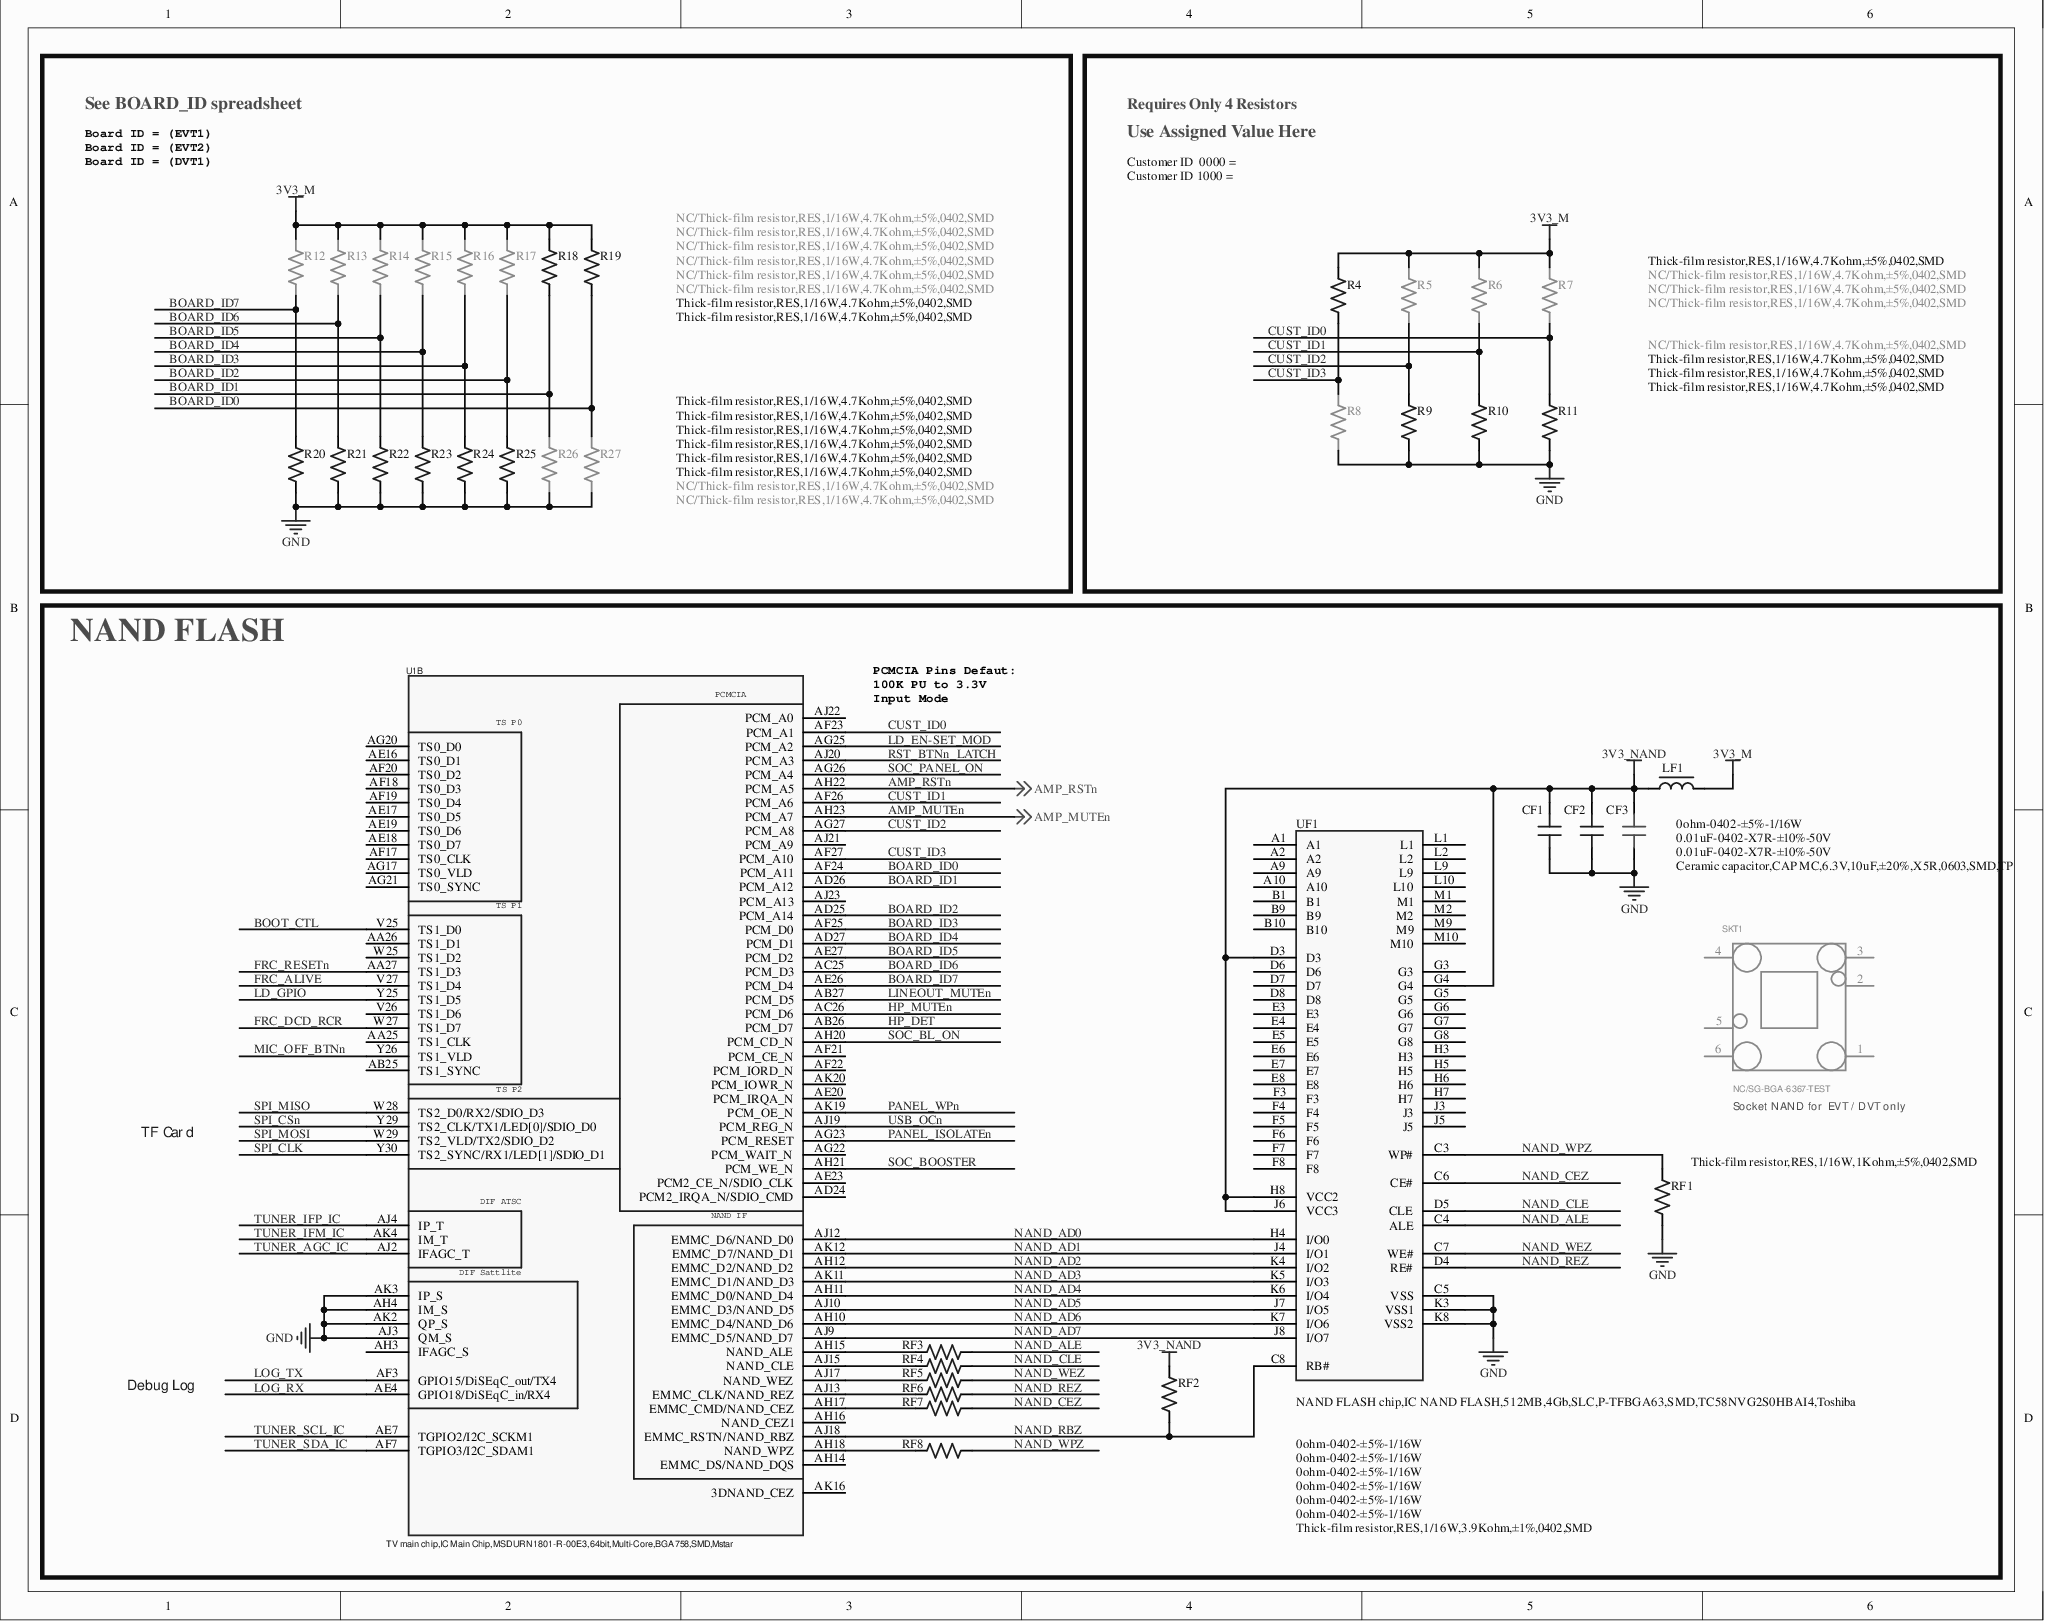
[diagram p0: MISC86290-10.SchDoc]
# Altium project MISC86290.PrjPcb (part 8 of 13)

## Sheet MISC86290-10.SchDoc
size 368 x 292 mm

### Parts
CF1  0.01uF-0402-X7R-±10%-50V  [C0402]
CF2  0.01uF-0402-X7R-±10%-50V  [C0402]
CF3  Ceramic capacitor,CAP MC,6.3V,10uF,±20%,X5R,0603,SMD,TP  [C0603]
LF1  0ohm-0402-±5%-1/16W  [L0402]
R4  Thick-film resistor,RES,1/16W,4.7Kohm,±5%,0402,SMD  [R0402]
R5  NC/Thick-film resistor,RES,1/16W,4.7Kohm,±5%,0402,SMD  [R0402]
R6  NC/Thick-film resistor,RES,1/16W,4.7Kohm,±5%,0402,SMD  [R0402]
R7  NC/Thick-film resistor,RES,1/16W,4.7Kohm,±5%,0402,SMD  [R0402]
R8  NC/Thick-film resistor,RES,1/16W,4.7Kohm,±5%,0402,SMD  [R0402]
R9  Thick-film resistor,RES,1/16W,4.7Kohm,±5%,0402,SMD  [R0402]
R10  Thick-film resistor,RES,1/16W,4.7Kohm,±5%,0402,SMD  [R0402]
R11  Thick-film resistor,RES,1/16W,4.7Kohm,±5%,0402,SMD  [R0402]
R12  NC/Thick-film resistor,RES,1/16W,4.7Kohm,±5%,0402,SMD  [R0402]
R13  NC/Thick-film resistor,RES,1/16W,4.7Kohm,±5%,0402,SMD  [R0402]
R14  NC/Thick-film resistor,RES,1/16W,4.7Kohm,±5%,0402,SMD  [R0402]
R15  NC/Thick-film resistor,RES,1/16W,4.7Kohm,±5%,0402,SMD  [R0402]
R16  NC/Thick-film resistor,RES,1/16W,4.7Kohm,±5%,0402,SMD  [R0402]
R17  NC/Thick-film resistor,RES,1/16W,4.7Kohm,±5%,0402,SMD  [R0402]
R18  Thick-film resistor,RES,1/16W,4.7Kohm,±5%,0402,SMD  [R0402]
R19  Thick-film resistor,RES,1/16W,4.7Kohm,±5%,0402,SMD  [R0402]
R20  Thick-film resistor,RES,1/16W,4.7Kohm,±5%,0402,SMD  [R0402]
R21  Thick-film resistor,RES,1/16W,4.7Kohm,±5%,0402,SMD  [R0402]
R22  Thick-film resistor,RES,1/16W,4.7Kohm,±5%,0402,SMD  [R0402]
R23  Thick-film resistor,RES,1/16W,4.7Kohm,±5%,0402,SMD  [R0402]
R24  Thick-film resistor,RES,1/16W,4.7Kohm,±5%,0402,SMD  [R0402]
R25  Thick-film resistor,RES,1/16W,4.7Kohm,±5%,0402,SMD  [R0402]
R26  NC/Thick-film resistor,RES,1/16W,4.7Kohm,±5%,0402,SMD  [R0402]
R27  NC/Thick-film resistor,RES,1/16W,4.7Kohm,±5%,0402,SMD  [R0402]
RF1  Thick-film resistor,RES,1/16W,1Kohm,±5%,0402,SMD  [R0402]
RF2  Thick-film resistor,RES,1/16W,3.9Kohm,±1%,0402,SMD  [R0402]
RF3  0ohm-0402-±5%-1/16W  [R0402]
RF4  0ohm-0402-±5%-1/16W  [R0402]
RF5  0ohm-0402-±5%-1/16W  [R0402]
RF6  0ohm-0402-±5%-1/16W  [R0402]
RF7  0ohm-0402-±5%-1/16W  [R0402]
RF8  0ohm-0402-±5%-1/16W  [R0402]
SKT1  NC/SG-BGA-6367-TEST  [TEST-SG-BGA-6367]
U1  TV main chip,IC Main Chip,MSDURN1801-R-00E3,64bit,Multi-Core,BGA758,SMD,Mstar  [BGA758/0.65]  (part B of 7)
UF1  NAND FLASH chip,IC NAND FLASH,512MB,4Gb,SLC,P-TFBGA63,SMD,TC58NVG2S0HBAI4,Toshiba  [BGA63/0.8-1]

### Blocks framed on the sheet
See BOARD_ID spreadsheet: R12-R27
Use Assigned Value Here: R4-R11
NAND FLASH: CF1-CF3 LF1 RF1-RF8 SKT1 U1 UF1

### Nets
3V3_M: LF1.2 R4.2 R5.2 R6.2 R7.2 R12.2 R13.2 R14.2 R15.2 R16.2 R17.2 R18.2 R19.2
3V3_NAND: CF1.2 CF2.2 CF3.2 LF1.1 RF2.2 UF1.D3 UF1.G4 UF1.H8(VCC2) UF1.J6(VCC3)
GND: CF1.1 CF2.1 CF3.1 R8.1 R9.1 R10.1 R11.1 R20.1 R21.1 R22.1 R23.1 R24.1 R25.1 R26.1 R27.1 RF1.1 U1.AH4(IM_S) U1.AJ3(QM_S) U1.AK2(QP_S) U1.AK3(IP_S) UF1.C5(VSS) UF1.K3(VSS1) UF1.K8(VSS2)
AMP_MUTEn: U1.AH23(PCM_A7) ; off-sheet AMP_MUTEn
AMP_RSTn: U1.AH22(PCM_A5) ; off-sheet AMP_RSTn
BOARD_ID0: R19.1 R27.2 U1.AF24(PCM_A11)
BOARD_ID1: R18.1 R26.2 U1.AD26(PCM_A12)
BOARD_ID2: R17.1 R25.2 U1.AD25(PCM_A14)
BOARD_ID3: R16.1 R24.2 U1.AF25(PCM_D0)
BOARD_ID4: R15.1 R23.2 U1.AD27(PCM_D1)
BOARD_ID5: R14.1 R22.2 U1.AE27(PCM_D2)
BOARD_ID6: R13.1 R21.2 U1.AC25(PCM_D3)
BOARD_ID7: R12.1 R20.2 U1.AE26(PCM_D4)
BOOT_CTL: U1.V25(TS1_D0)
CUST_ID0: R7.1 R11.2 U1.AF23(PCM_A1)
CUST_ID1: R6.1 R10.2 U1.AF26(PCM_A6)
CUST_ID2: R5.1 R9.2 U1.AG27(PCM_A8)
CUST_ID3: R4.1 R8.2 U1.AF27(PCM_A10)
FRC_ALIVE: U1.V27(TS1_D4)
FRC_DCD_RCR: U1.W27(TS1_D7)
FRC_RESETn: U1.AA27(TS1_D3)
HP_DET: U1.AB26(PCM_D7)
HP_MUTEn: U1.AC26(PCM_D6)
LD_EN-SET_MOD: U1.AG25(PCM_A2)
LD_GPIO: U1.Y25(TS1_D5)
LINEOUT_MUTEn: U1.AB27(PCM_D5)
LOG_RX: U1.AE4(GPIO18/DiSEqC_in/RX4)
LOG_TX: U1.AF3(GPIO15/DiSEqC_out/TX4)
MIC_OFF_BTNn: U1.Y26(TS1_VLD)
NAND_AD0: U1.AJ12(EMMC_D6/NAND_D0) UF1.H4(I/O0)
NAND_AD1: U1.AK12(EMMC_D7/NAND_D1) UF1.J4(I/O1)
NAND_AD2: U1.AH12(EMMC_D2/NAND_D2) UF1.K4(I/O2)
NAND_AD3: U1.AK11(EMMC_D1/NAND_D3) UF1.K5(I/O3)
NAND_AD4: U1.AH11(EMMC_D0/NAND_D4) UF1.K6(I/O4)
NAND_AD5: U1.AJ10(EMMC_D3/NAND_D5) UF1.J7(I/O5)
NAND_AD6: U1.AH10(EMMC_D4/NAND_D6) UF1.K7(I/O6)
NAND_AD7: U1.AJ9(EMMC_D5/NAND_D7) UF1.J8(I/O7)
NAND_ALE: RF3.2 UF1.C4(ALE)
NAND_CEZ: RF7.2 UF1.C6(CE#)
NAND_CLE: RF4.2 UF1.D5(CLE)
NAND_RBZ: RF2.1 U1.AJ18(EMMC_RSTN/NAND_RBZ) UF1.C8(RB#)
NAND_REZ: RF6.2 UF1.D4(RE#)
NAND_WEZ: RF5.2 UF1.C7(WE#)
NAND_WPZ: RF1.2 RF8.2 UF1.C3(WP#)
PANEL_ISOLATEn: U1.AG23(PCM_RESET)
PANEL_WPn: U1.AK19(PCM_OE_N)
RST_BTNn_LATCH: U1.AJ20(PCM_A3)
SOC_BL_ON: U1.AH20(PCM_CD_N)
SOC_BOOSTER: U1.AH21(PCM_WE_N)
SOC_PANEL_ON: U1.AG26(PCM_A4)
SPI_CLK: U1.Y30(TS2_SYNC/RX1/LED[1]/SDIO_D1)
SPI_CSn: U1.Y29(TS2_CLK/TX1/LED[0]/SDIO_D0)
SPI_MISO: U1.W28(TS2_D0/RX2/SDIO_D3)
SPI_MOSI: U1.W29(TS2_VLD/TX2/SDIO_D2)
TUNER_AGC_IC: U1.AJ2(IFAGC_T)
TUNER_IFM_IC: U1.AK4(IM_T)
TUNER_IFP_IC: U1.AJ4(IP_T)
TUNER_SCL_IC: U1.AE7(TGPIO2/I2C_SCKM1)
TUNER_SDA_IC: U1.AF7(TGPIO3/I2C_SDAM1)
USB_OCn: U1.AJ19(PCM_REG_N)
NetRF3_1: RF3.1 U1.AH15(NAND_ALE)
NetRF4_1: RF4.1 U1.AJ15(NAND_CLE)
NetRF5_1: RF5.1 U1.AJ17(NAND_WEZ)
NetRF6_1: RF6.1 U1.AJ13(EMMC_CLK/NAND_REZ)
NetRF7_1: RF7.1 U1.AH17(EMMC_CMD/NAND_CEZ)
NetRF8_1: RF8.1 U1.AH18(NAND_WPZ)

Not connected (* = marked no-connect by the designer): SKT1 1* 2* 3* 4* 5* 6*; U1 AA25(TS1_CLK)* AA26(TS1_D1)* AB25(TS1_SYNC)* AD24(PCM2_IRQA_N/SDIO_CMD)* AE16(TS0_D1)* AE17(TS0_D5)* AE18(TS0_D7)* AE19(TS0_D6)* AE20(PCM_IRQA_N)* AE23(PCM2_CE_N/SDIO_CLK)* AF17(TS0_CLK)* AF18(TS0_D3)* AF19(TS0_D4)* AF20(TS0_D2)* AF21(PCM_CE_N)* AF22(PCM_IORD_N)* AG17(TS0_VLD)* AG20(TS0_D0)* AG21(TS0_SYNC)* AG22(PCM_WAIT_N)* AH3(IFAGC_S)* AH14(EMMC_DS/NAND_DQS)* AH16(NAND_CEZ1)* AJ21(PCM_A9)* AJ22(PCM_A0)* AJ23(PCM_A13)* AK16(3DNAND_CEZ)* AK20(PCM_IOWR_N)* V26(TS1_D6)* W25(TS1_D2)*; UF1 A1* A2* A9* A10* B1* B9* B10* D6* D7* D8* E3* E4* E5* E6* E7* E8* F3* F4* F5* F6* F7* F8* G3* G5* G6* G7* G8* H3* H5* H6* H7* J3* J5* L1* L2* L9* L10* M1* M2* M9* M10*

### Notes on the sheet
- Board ID = (EVT1)
- Board ID = (EVT2)
- Board ID = (DVT1)
- Requires Only 4 Resistors
- Customer ID  0000 = (COMPANY_B)
- Customer ID 1000 = (COMPANY_A)
- PCMCIA Pins Defaut:
  100K PU to 3.3V
  Input Mode
- TF Card
- (near SKT1) Socket NAND for  EVT / DVT only
- Debug Log

### Library data of the parts
CF1 CF2 = 004.003.0000505-D: Ceramic capacitor,CAP MC,16V,0.01uF,±10%,X7R,0402,SMD,TP-D
CF3 = 004.003.0000383-D: Ceramic capacitor,CAP MC,6.3V,10uF,±20%,X5R,0603,SMD,TP-D
LF1 = HCB1005KF-121T20(120ohm-1200mA)-D
R4-R27 = 004.002.0000689-D: Thick-film resistor,RES,1/16W,4.7Kohm,±5%,0402,SMD-D
RF1 = 004.002.0000572-D: Thick-film resistor,RES,1/16W,1Kohm,±5%,0402,SMD-D
RF2 = 004.002.0000675-D: Thick-film resistor,RES,1/16W,3.9Kohm,±1%,0402,SMD-D
RF3-RF8 = 0ohm-0402-±5%-1/16W-D
SKT1 = SG-BGA-6367-TEST: SG-BGA-6367 test socket
U1 = 004.016.0001110-D: TV main chip,IC Main Chip,MSDURN1801-Z1,64bit,Multi-Core,BGA758,SMD,Mstar-D
UF1 = PKG-003578/P000079162: NAND FLASH chip,512MB,4Gb,TC58NVG2S0HBAI4,TOSHIBA-D

## Sheet MISC86290-11.SchDoc
size 754 x 292 mm
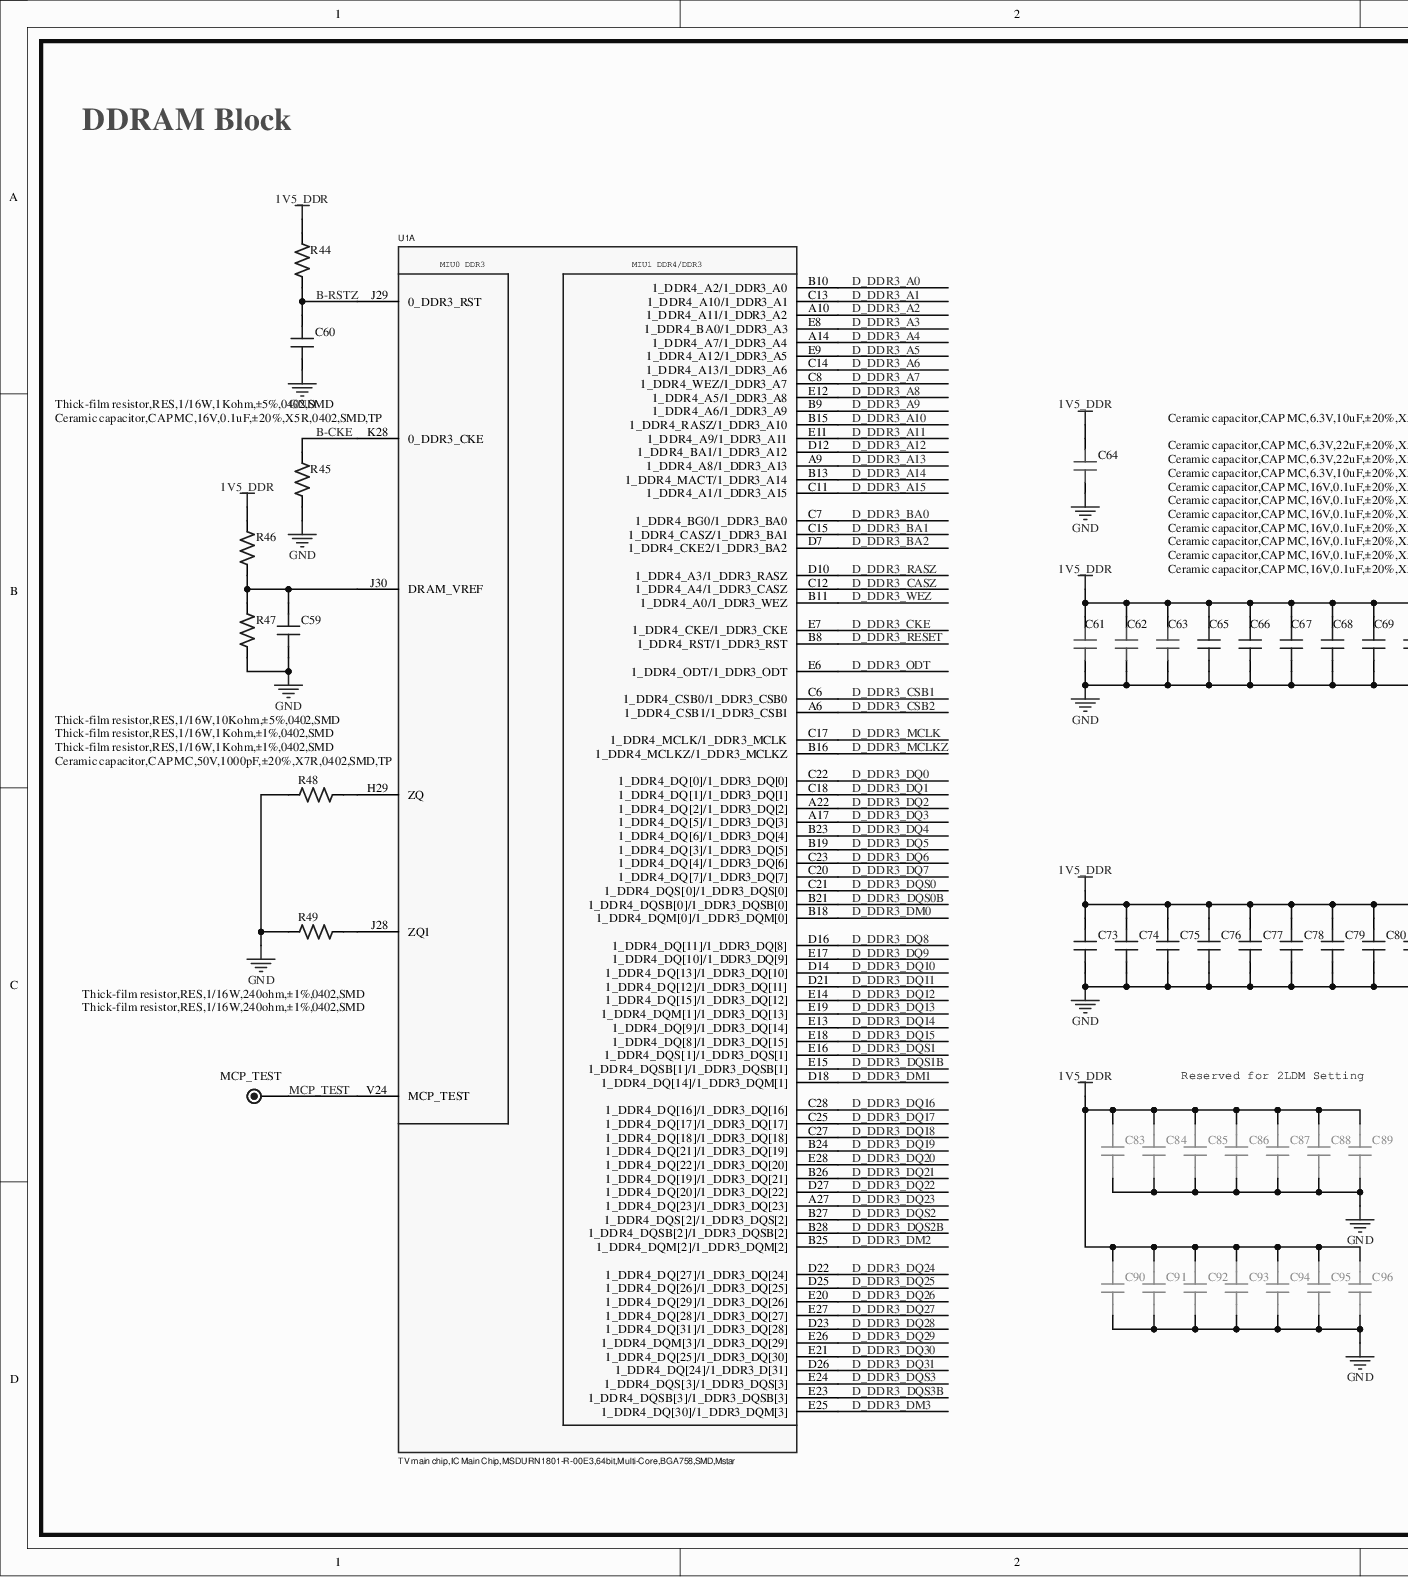
[diagram p1: MISC86290-11.SchDoc, left]
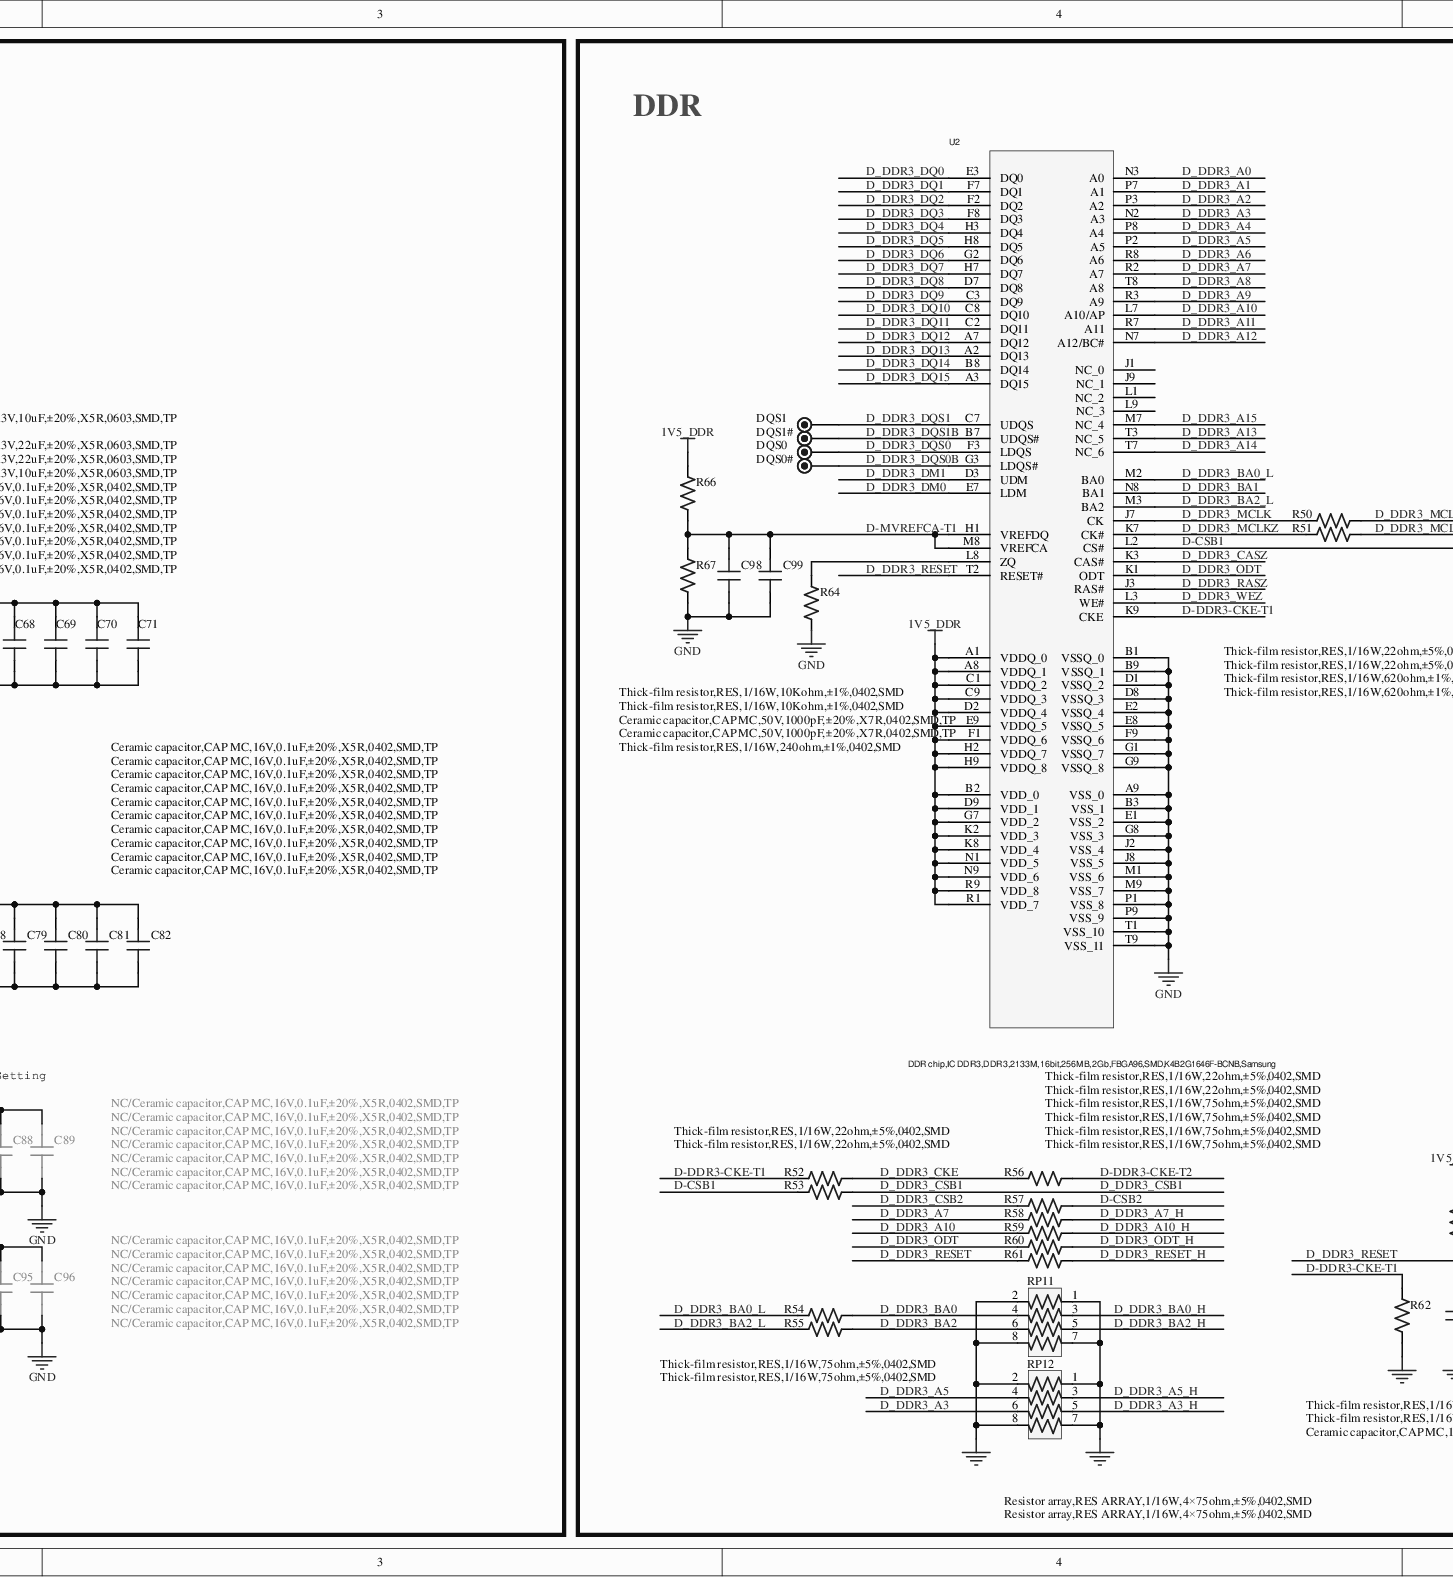
[diagram p2: MISC86290-11.SchDoc, middle]
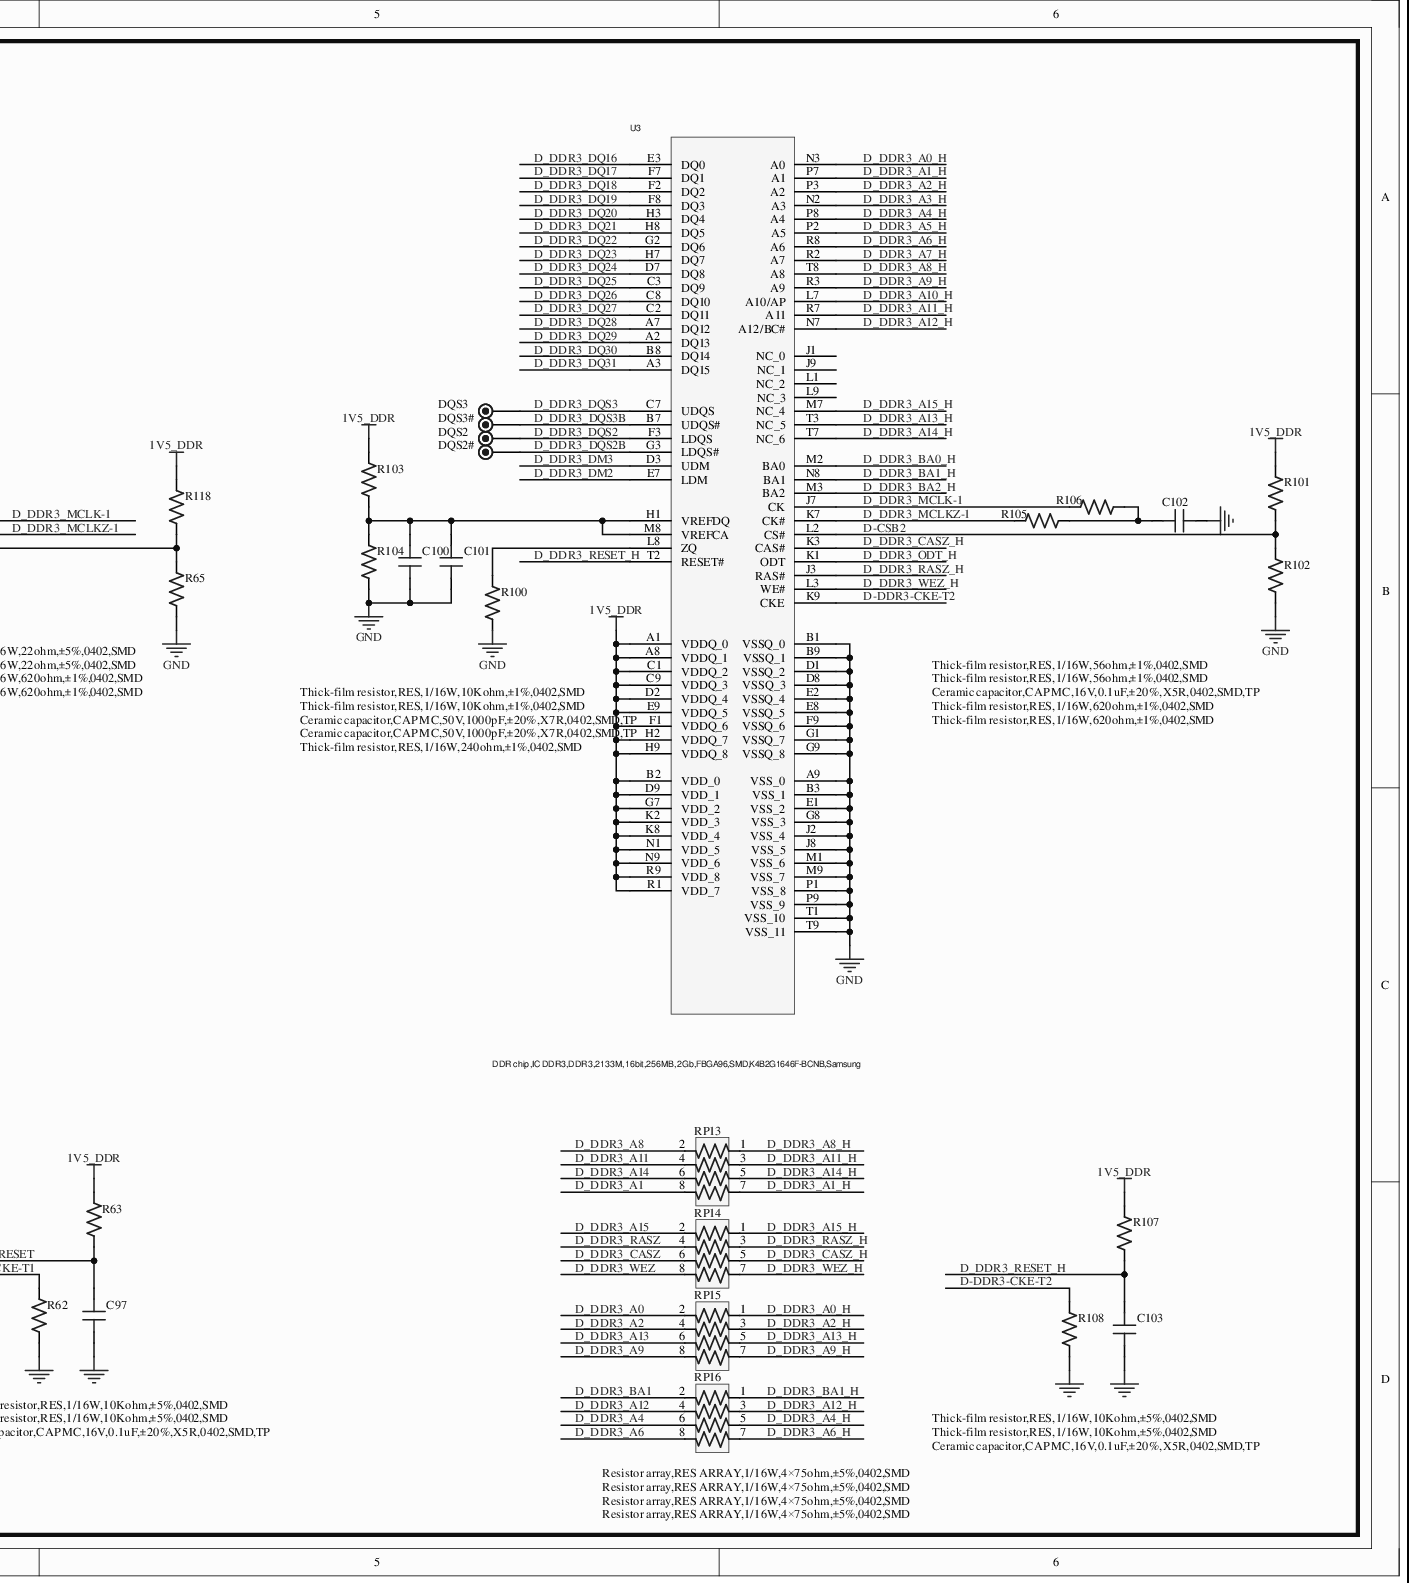
[diagram p3: MISC86290-11.SchDoc, right]

### Parts
C59  Ceramic capacitor,CAP MC,50V,1000pF,±20%,X7R,0402,SMD,TP  [C0402]
C60  Ceramic capacitor,CAP MC,16V,0.1uF,±20%,X5R,0402,SMD,TP  [C0402]
C61  Ceramic capacitor,CAP MC,6.3V,22uF,±20%,X5R,0603,SMD,TP  [C0603]
C62  Ceramic capacitor,CAP MC,6.3V,22uF,±20%,X5R,0603,SMD,TP  [C0603]
C63  Ceramic capacitor,CAP MC,6.3V,10uF,±20%,X5R,0603,SMD,TP  [C0603]
C64  Ceramic capacitor,CAP MC,6.3V,10uF,±20%,X5R,0603,SMD,TP  [C0603]
C65  Ceramic capacitor,CAP MC,16V,0.1uF,±20%,X5R,0402,SMD,TP  [C0402]
C66  Ceramic capacitor,CAP MC,16V,0.1uF,±20%,X5R,0402,SMD,TP  [C0402]
C67  Ceramic capacitor,CAP MC,16V,0.1uF,±20%,X5R,0402,SMD,TP  [C0402]
C68  Ceramic capacitor,CAP MC,16V,0.1uF,±20%,X5R,0402,SMD,TP  [C0402]
C69  Ceramic capacitor,CAP MC,16V,0.1uF,±20%,X5R,0402,SMD,TP  [C0402]
C70  Ceramic capacitor,CAP MC,16V,0.1uF,±20%,X5R,0402,SMD,TP  [C0402]
C71  Ceramic capacitor,CAP MC,16V,0.1uF,±20%,X5R,0402,SMD,TP  [C0402]
C73  Ceramic capacitor,CAP MC,16V,0.1uF,±20%,X5R,0402,SMD,TP  [C0402]
C74  Ceramic capacitor,CAP MC,16V,0.1uF,±20%,X5R,0402,SMD,TP  [C0402]
C75  Ceramic capacitor,CAP MC,16V,0.1uF,±20%,X5R,0402,SMD,TP  [C0402]
C76  Ceramic capacitor,CAP MC,16V,0.1uF,±20%,X5R,0402,SMD,TP  [C0402]
C77  Ceramic capacitor,CAP MC,16V,0.1uF,±20%,X5R,0402,SMD,TP  [C0402]
C78  Ceramic capacitor,CAP MC,16V,0.1uF,±20%,X5R,0402,SMD,TP  [C0402]
C79  Ceramic capacitor,CAP MC,16V,0.1uF,±20%,X5R,0402,SMD,TP  [C0402]
C80  Ceramic capacitor,CAP MC,16V,0.1uF,±20%,X5R,0402,SMD,TP  [C0402]
C81  Ceramic capacitor,CAP MC,16V,0.1uF,±20%,X5R,0402,SMD,TP  [C0402]
C82  Ceramic capacitor,CAP MC,16V,0.1uF,±20%,X5R,0402,SMD,TP  [C0402]
C83  NC/Ceramic capacitor,CAP MC,16V,0.1uF,±20%,X5R,0402,SMD,TP  [C0402]
C84  NC/Ceramic capacitor,CAP MC,16V,0.1uF,±20%,X5R,0402,SMD,TP  [C0402]
C85  NC/Ceramic capacitor,CAP MC,16V,0.1uF,±20%,X5R,0402,SMD,TP  [C0402]
C86  NC/Ceramic capacitor,CAP MC,16V,0.1uF,±20%,X5R,0402,SMD,TP  [C0402]
C87  NC/Ceramic capacitor,CAP MC,16V,0.1uF,±20%,X5R,0402,SMD,TP  [C0402]
C88  NC/Ceramic capacitor,CAP MC,16V,0.1uF,±20%,X5R,0402,SMD,TP  [C0402]
C89  NC/Ceramic capacitor,CAP MC,16V,0.1uF,±20%,X5R,0402,SMD,TP  [C0402]
C90  NC/Ceramic capacitor,CAP MC,16V,0.1uF,±20%,X5R,0402,SMD,TP  [C0402]
C91  NC/Ceramic capacitor,CAP MC,16V,0.1uF,±20%,X5R,0402,SMD,TP  [C0402]
C92  NC/Ceramic capacitor,CAP MC,16V,0.1uF,±20%,X5R,0402,SMD,TP  [C0402]
C93  NC/Ceramic capacitor,CAP MC,16V,0.1uF,±20%,X5R,0402,SMD,TP  [C0402]
C94  NC/Ceramic capacitor,CAP MC,16V,0.1uF,±20%,X5R,0402,SMD,TP  [C0402]
C95  NC/Ceramic capacitor,CAP MC,16V,0.1uF,±20%,X5R,0402,SMD,TP  [C0402]
C96  NC/Ceramic capacitor,CAP MC,16V,0.1uF,±20%,X5R,0402,SMD,TP  [C0402]
C97  Ceramic capacitor,CAP MC,16V,0.1uF,±20%,X5R,0402,SMD,TP  [C0402]
C98  Ceramic capacitor,CAP MC,50V,1000pF,±20%,X7R,0402,SMD,TP  [C0402]
C99  Ceramic capacitor,CAP MC,50V,1000pF,±20%,X7R,0402,SMD,TP  [C0402]
C100  Ceramic capacitor,CAP MC,50V,1000pF,±20%,X7R,0402,SMD,TP  [C0402]
C101  Ceramic capacitor,CAP MC,50V,1000pF,±20%,X7R,0402,SMD,TP  [C0402]
C102  Ceramic capacitor,CAP MC,16V,0.1uF,±20%,X5R,0402,SMD,TP  [C0402]
C103  Ceramic capacitor,CAP MC,16V,0.1uF,±20%,X5R,0402,SMD,TP  [C0402]
DQS0  TEST  [TP-20]  (value not drawn)
DQS0#  TEST  [TP-20]  (value not drawn)
DQS1  TEST  [TP-20]  (value not drawn)
DQS1#  TEST  [TP-20]  (value not drawn)
DQS2  TEST  [TP-20]  (value not drawn)
DQS2#  TEST  [TP-20]  (value not drawn)
DQS3  TEST  [TP-20]  (value not drawn)
DQS3#  TEST  [TP-20]  (value not drawn)
MCP_TEST  TEST  [TP-20]  (value not drawn)
R44  Thick-film resistor,RES,1/16W,1Kohm,±5%,0402,SMD  [R0402]
R45  Thick-film resistor,RES,1/16W,10Kohm,±5%,0402,SMD  [R0402]
R46  Thick-film resistor,RES,1/16W,1Kohm,±1%,0402,SMD  [R0402]
R47  Thick-film resistor,RES,1/16W,1Kohm,±1%,0402,SMD  [R0402]
R48  Thick-film resistor,RES,1/16W,240ohm,±1%,0402,SMD  [R0402]
R49  Thick-film resistor,RES,1/16W,240ohm,±1%,0402,SMD  [R0402]
R50  Thick-film resistor,RES,1/16W,22ohm,±5%,0402,SMD  [R0402]
R51  Thick-film resistor,RES,1/16W,22ohm,±5%,0402,SMD  [R0402]
R52  Thick-film resistor,RES,1/16W,22ohm,±5%,0402,SMD  [R0402]
R53  Thick-film resistor,RES,1/16W,22ohm,±5%,0402,SMD  [R0402]
R54  Thick-film resistor,RES,1/16W,75ohm,±5%,0402,SMD  [R0402]
R55  Thick-film resistor,RES,1/16W,75ohm,±5%,0402,SMD  [R0402]
R56  Thick-film resistor,RES,1/16W,22ohm,±5%,0402,SMD  [R0402]
R57  Thick-film resistor,RES,1/16W,22ohm,±5%,0402,SMD  [R0402]
R58  Thick-film resistor,RES,1/16W,75ohm,±5%,0402,SMD  [R0402]
R59  Thick-film resistor,RES,1/16W,75ohm,±5%,0402,SMD  [R0402]
R60  Thick-film resistor,RES,1/16W,75ohm,±5%,0402,SMD  [R0402]
R61  Thick-film resistor,RES,1/16W,75ohm,±5%,0402,SMD  [R0402]
R62  Thick-film resistor,RES,1/16W,10Kohm,±5%,0402,SMD  [R0402]
R63  Thick-film resistor,RES,1/16W,10Kohm,±5%,0402,SMD  [R0402]
R64  Thick-film resistor,RES,1/16W,240ohm,±1%,0402,SMD  [R0402]
R65  Thick-film resistor,RES,1/16W,620ohm,±1%,0402,SMD  [R0402]
R66  Thick-film resistor,RES,1/16W,10Kohm,±1%,0402,SMD  [R0402]
R67  Thick-film resistor,RES,1/16W,10Kohm,±1%,0402,SMD  [R0402]
R100  Thick-film resistor,RES,1/16W,240ohm,±1%,0402,SMD  [R0402]
R101  Thick-film resistor,RES,1/16W,620ohm,±1%,0402,SMD  [R0402]
R102  Thick-film resistor,RES,1/16W,620ohm,±1%,0402,SMD  [R0402]
R103  Thick-film resistor,RES,1/16W,10Kohm,±1%,0402,SMD  [R0402]
R104  Thick-film resistor,RES,1/16W,10Kohm,±1%,0402,SMD  [R0402]
R105  Thick-film resistor,RES,1/16W,56ohm,±1%,0402,SMD  [R0402]
R106  Thick-film resistor,RES,1/16W,56ohm,±1%,0402,SMD  [R0402]
R107  Thick-film resistor,RES,1/16W,10Kohm,±5%,0402,SMD  [R0402]
R108  Thick-film resistor,RES,1/16W,10Kohm,±5%,0402,SMD  [R0402]
R118  Thick-film resistor,RES,1/16W,620ohm,±1%,0402,SMD  [R0402]
RP11  Resistor array,RES ARRAY,1/16W,4×75ohm,±5%,0402,SMD  [RA0402-MSD6886]
RP12  Resistor array,RES ARRAY,1/16W,4×75ohm,±5%,0402,SMD  [RA0402-MSD6886]
RP13  Resistor array,RES ARRAY,1/16W,4×75ohm,±5%,0402,SMD  [RA0402-MSD6886]
RP14  Resistor array,RES ARRAY,1/16W,4×75ohm,±5%,0402,SMD  [RA0402-MSD6886]
RP15  Resistor array,RES ARRAY,1/16W,4×75ohm,±5%,0402,SMD  [RA0402-MSD6886]
RP16  Resistor array,RES ARRAY,1/16W,4×75ohm,±5%,0402,SMD  [RA0402-MSD6886]
U1  TV main chip,IC Main Chip,MSDURN1801-R-00E3,64bit,Multi-Core,BGA758,SMD,Mstar  [BGA758/0.65]  (part A of 7)
U2  DDR chip,IC DDR3,DDR3,2133M,16bit,256MB,2Gb,FBGA96,SMD,K4B2G1646F-BCNB,Samsung  [BGA96/0.8-1]
U3  DDR chip,IC DDR3,DDR3,2133M,16bit,256MB,2Gb,FBGA96,SMD,K4B2G1646F-BCNB,Samsung  [BGA96/0.8-1]

### Blocks framed on the sheet
DDRAM Block: C59-C71 C73-C96 MCP_TEST R44-R49 U1
DDR: C97-C103 DQS0 DQS0# DQS1 DQS1# DQS2 DQS2# DQS3 DQS3# R50-R67 R100-R108 R118 RP11-RP16 U2 U3

### Nets
1V5_DDR: C61.2 C62.2 C63.2 C64.2 C65.2 C66.2 C67.2 C68.2 C69.2 C70.2 C71.2 C73.2 C74.2 C75.2 C76.2 C77.2 C78.2 C79.2 C80.2 C81.2 C82.2 C83.2 C84.2 C85.2 C86.2 C87.2 C88.2 C89.2 C90.2 C91.2 C92.2 C93.2 C94.2 C95.2 C96.2 R44.2 R46.2 R63.2 R66.2 R101.2 R103.2 R107.2 R118.2 U2.A1(VDDQ_0) U2.A8(VDDQ_1) U2.B2(VDD_0) U2.C1(VDDQ_2) U2.C9(VDDQ_3) U2.D2(VDDQ_4) U2.D9(VDD_1) U2.E9(VDDQ_5) U2.F1(VDDQ_6) U2.G7(VDD_2) U2.H2(VDDQ_7) U2.H9(VDDQ_8) U2.K2(VDD_3) U2.K8(VDD_4) U2.N1(VDD_5) U2.N9(VDD_6) U2.R1(VDD_7) U2.R9(VDD_8) U3.A1(VDDQ_0) U3.A8(VDDQ_1) U3.B2(VDD_0) U3.C1(VDDQ_2) U3.C9(VDDQ_3) U3.D2(VDDQ_4) U3.D9(VDD_1) U3.E9(VDDQ_5) U3.F1(VDDQ_6) U3.G7(VDD_2) U3.H2(VDDQ_7) U3.H9(VDDQ_8) U3.K2(VDD_3) U3.K8(VDD_4) U3.N1(VDD_5) U3.N9(VDD_6) U3.R1(VDD_7) U3.R9(VDD_8)
GND: C59.1 C60.1 C61.1 C62.1 C63.1 C64.1 C65.1 C66.1 C67.1 C68.1 C69.1 C70.1 C71.1 C73.1 C74.1 C75.1 C76.1 C77.1 C78.1 C79.1 C80.1 C81.1 C82.1 C83.1 C84.1 C85.1 C86.1 C87.1 C88.1 C89.1 C90.1 C91.1 C92.1 C93.1 C94.1 C95.1 C96.1 C97.1 C98.1 C99.1 C100.1 C101.1 C102.1 C103.1 R45.1 R47.1 R48.1 R49.1 R62.1 R64.1 R65.1 R67.1 R100.1 R102.1 R104.1 R108.1 RP11.1 RP11.2 RP11.7 RP11.8 RP12.1 RP12.2 RP12.7 RP12.8 U2.A9(VSS_0) U2.B1(VSSQ_0) U2.B3(VSS_1) U2.B9(VSSQ_1) U2.D1(VSSQ_2) U2.D8(VSSQ_3) U2.E1(VSS_2) U2.E2(VSSQ_4) U2.E8(VSSQ_5) U2.F9(VSSQ_6) U2.G1(VSSQ_7) U2.G8(VSS_3) U2.G9(VSSQ_8) U2.J2(VSS_4) U2.J8(VSS_5) U2.M1(VSS_6) U2.M9(VSS_7) U2.P1(VSS_8) U2.P9(VSS_9) U2.T1(VSS_10) U2.T9(VSS_11) U3.A9(VSS_0) U3.B1(VSSQ_0) U3.B3(VSS_1) U3.B9(VSSQ_1) U3.D1(VSSQ_2) U3.D8(VSSQ_3) U3.E1(VSS_2) U3.E2(VSSQ_4) U3.E8(VSSQ_5) U3.F9(VSSQ_6) U3.G1(VSSQ_7) U3.G8(VSS_3) U3.G9(VSSQ_8) U3.J2(VSS_4) U3.J8(VSS_5) U3.M1(VSS_6) U3.M9(VSS_7) U3.P1(VSS_8) U3.P9(VSS_9) U3.T1(VSS_10) U3.T9(VSS_11)
B-CKE: R45.2 U1.K28(0_DDR3_CKE)
B-RSTZ: C60.2 R44.1 U1.J29(0_DDR3_RST)
D-CSB1: R53.1 R65.2 R118.1 U2.L2(CS#)
D-CSB2: R57.2 R101.1 R102.2 U3.L2(CS#)
D-DDR3-CKE-T1: R52.1 R62.2 U2.K9(CKE)
D-DDR3-CKE-T2: R56.2 R108.2 U3.K9(CKE)
D-MVREFCA-T1: C98.2 C99.2 R66.1 R67.2 U2.H1(VREFDQ) U2.M8(VREFCA)
D_DDR3_A0: RP15.2 U1.B10(1_DDR4_A2/1_DDR3_A0) U2.N3(A0)
D_DDR3_A0_H: RP15.1 U3.N3(A0)
D_DDR3_A1: RP13.8 U1.C13(1_DDR4_A10/1_DDR3_A1) U2.P7(A1)
D_DDR3_A1_H: RP13.7 U3.P7(A1)
D_DDR3_A2: RP15.4 U1.A10(1_DDR4_A11/1_DDR3_A2) U2.P3(A2)
D_DDR3_A2_H: RP15.3 U3.P3(A2)
D_DDR3_A3: RP12.6 U1.E8(1_DDR4_BA0/1_DDR3_A3) U2.N2(A3)
D_DDR3_A3_H: RP12.5 U3.N2(A3)
D_DDR3_A4: RP16.6 U1.A14(1_DDR4_A7/1_DDR3_A4) U2.P8(A4)
D_DDR3_A4_H: RP16.5 U3.P8(A4)
D_DDR3_A5: RP12.4 U1.E9(1_DDR4_A12/1_DDR3_A5) U2.P2(A5)
D_DDR3_A5_H: RP12.3 U3.P2(A5)
D_DDR3_A6: RP16.8 U1.C14(1_DDR4_A13/1_DDR3_A6) U2.R8(A6)
D_DDR3_A6_H: RP16.7 U3.R8(A6)
D_DDR3_A7: R58.1 U1.C8(1_DDR4_WEZ/1_DDR3_A7) U2.R2(A7)
D_DDR3_A7_H: R58.2 U3.R2(A7)
D_DDR3_A8: RP13.2 U1.E12(1_DDR4_A5/1_DDR3_A8) U2.T8(A8)
D_DDR3_A8_H: RP13.1 U3.T8(A8)
D_DDR3_A9: RP15.8 U1.B9(1_DDR4_A6/1_DDR3_A9) U2.R3(A9)
D_DDR3_A9_H: RP15.7 U3.R3(A9)
D_DDR3_A10: R59.1 U1.B15(1_DDR4_RASZ/1_DDR3_A10) U2.L7(A10/AP)
D_DDR3_A10_H: R59.2 U3.L7(A10/AP)
D_DDR3_A11: RP13.4 U1.E11(1_DDR4_A9/1_DDR3_A11) U2.R7(A11)
D_DDR3_A11_H: RP13.3 U3.R7(A11)
D_DDR3_A12: RP16.4 U1.D12(1_DDR4_BA1/1_DDR3_A12) U2.N7(A12/BC#)
D_DDR3_A12_H: RP16.3 U3.N7(A12/BC#)
D_DDR3_A13: RP15.6 U1.A9(1_DDR4_A8/1_DDR3_A13) U2.T3(NC_5)
D_DDR3_A13_H: RP15.5 U3.T3(NC_5)
D_DDR3_A14: RP13.6 U1.B13(1_DDR4_MACT/1_DDR3_A14) U2.T7(NC_6)
D_DDR3_A14_H: RP13.5 U3.T7(NC_6)
D_DDR3_A15: RP14.2 U1.C11(1_DDR4_A1/1_DDR3_A15) U2.M7(NC_4)
D_DDR3_A15_H: RP14.1 U3.M7(NC_4)
D_DDR3_BA0: R54.2 RP11.4 U1.C7(1_DDR4_BG0/1_DDR3_BA0)
D_DDR3_BA0_H: RP11.3 U3.M2(BA0)
D_DDR3_BA0_L: R54.1 U2.M2(BA0)
D_DDR3_BA1: RP16.2 U1.C15(1_DDR4_CASZ/1_DDR3_BA1) U2.N8(BA1)
D_DDR3_BA1_H: RP16.1 U3.N8(BA1)
D_DDR3_BA2: R55.2 RP11.6 U1.D7(1_DDR4_CKE2/1_DDR3_BA2)
D_DDR3_BA2_H: RP11.5 U3.M3(BA2)
D_DDR3_BA2_L: R55.1 U2.M3(BA2)
D_DDR3_CASZ: RP14.6 U1.C12(1_DDR4_A4/1_DDR3_CASZ) U2.K3(CAS#)
D_DDR3_CASZ_H: RP14.5 U3.K3(CAS#)
D_DDR3_CKE: R52.2 R56.1 U1.E7(1_DDR4_CKE/1_DDR3_CKE)
D_DDR3_CSB1: R53.2 U1.C6(1_DDR4_CSB0/1_DDR3_CSB0)
D_DDR3_CSB2: R57.1 U1.A6(1_DDR4_CSB1/1_DDR3_CSB1)
D_DDR3_DM0: U1.B18(1_DDR4_DQM[0]/1_DDR3_DQM[0]) U2.E7(LDM)
D_DDR3_DM1: U1.D18(1_DDR4_DQ[14]/1_DDR3_DQM[1]) U2.D3(UDM)
D_DDR3_DM2: U1.B25(1_DDR4_DQM[2]/1_DDR3_DQM[2]) U3.E7(LDM)
D_DDR3_DM3: U1.E25(1_DDR4_DQ[30]/1_DDR3_DQM[3]) U3.D3(UDM)
D_DDR3_DQ0: U1.C22(1_DDR4_DQ[0]/1_DDR3_DQ[0]) U2.E3(DQ0)
D_DDR3_DQ1: U1.C18(1_DDR4_DQ[1]/1_DDR3_DQ[1]) U2.F7(DQ1)
D_DDR3_DQ2: U1.A22(1_DDR4_DQ[2]/1_DDR3_DQ[2]) U2.F2(DQ2)
D_DDR3_DQ3: U1.A17(1_DDR4_DQ[5]/1_DDR3_DQ[3]) U2.F8(DQ3)
D_DDR3_DQ4: U1.B23(1_DDR4_DQ[6]/1_DDR3_DQ[4]) U2.H3(DQ4)
D_DDR3_DQ5: U1.B19(1_DDR4_DQ[3]/1_DDR3_DQ[5]) U2.H8(DQ5)
D_DDR3_DQ6: U1.C23(1_DDR4_DQ[4]/1_DDR3_DQ[6]) U2.G2(DQ6)
D_DDR3_DQ7: U1.C20(1_DDR4_DQ[7]/1_DDR3_DQ[7]) U2.H7(DQ7)
D_DDR3_DQ8: U1.D16(1_DDR4_DQ[11]/1_DDR3_DQ[8]) U2.D7(DQ8)
D_DDR3_DQ9: U1.E17(1_DDR4_DQ[10]/1_DDR3_DQ[9]) U2.C3(DQ9)
D_DDR3_DQ10: U1.D14(1_DDR4_DQ[13]/1_DDR3_DQ[10]) U2.C8(DQ10)
D_DDR3_DQ11: U1.D21(1_DDR4_DQ[12]/1_DDR3_DQ[11]) U2.C2(DQ11)
D_DDR3_DQ12: U1.E14(1_DDR4_DQ[15]/1_DDR3_DQ[12]) U2.A7(DQ12)
D_DDR3_DQ13: U1.E19(1_DDR4_DQM[1]/1_DDR3_DQ[13]) U2.A2(DQ13)
D_DDR3_DQ14: U1.E13(1_DDR4_DQ[9]/1_DDR3_DQ[14]) U2.B8(DQ14)
D_DDR3_DQ15: U1.E18(1_DDR4_DQ[8]/1_DDR3_DQ[15]) U2.A3(DQ15)
D_DDR3_DQ16: U1.C28(1_DDR4_DQ[16]/1_DDR3_DQ[16]) U3.E3(DQ0)
D_DDR3_DQ17: U1.C25(1_DDR4_DQ[17]/1_DDR3_DQ[17]) U3.F7(DQ1)
D_DDR3_DQ18: U1.C27(1_DDR4_DQ[18]/1_DDR3_DQ[18]) U3.F2(DQ2)
D_DDR3_DQ19: U1.B24(1_DDR4_DQ[21]/1_DDR3_DQ[19]) U3.F8(DQ3)
D_DDR3_DQ20: U1.E28(1_DDR4_DQ[22]/1_DDR3_DQ[20]) U3.H3(DQ4)
D_DDR3_DQ21: U1.B26(1_DDR4_DQ[19]/1_DDR3_DQ[21]) U3.H8(DQ5)
D_DDR3_DQ22: U1.D27(1_DDR4_DQ[20]/1_DDR3_DQ[22]) U3.G2(DQ6)
D_DDR3_DQ23: U1.A27(1_DDR4_DQ[23]/1_DDR3_DQ[23]) U3.H7(DQ7)
D_DDR3_DQ24: U1.D22(1_DDR4_DQ[27]/1_DDR3_DQ[24]) U3.D7(DQ8)
D_DDR3_DQ25: U1.D25(1_DDR4_DQ[26]/1_DDR3_DQ[25]) U3.C3(DQ9)
D_DDR3_DQ26: U1.E20(1_DDR4_DQ[29]/1_DDR3_DQ[26]) U3.C8(DQ10)
D_DDR3_DQ27: U1.E27(1_DDR4_DQ[28]/1_DDR3_DQ[27]) U3.C2(DQ11)
D_DDR3_DQ28: U1.D23(1_DDR4_DQ[31]/1_DDR3_DQ[28]) U3.A7(DQ12)
D_DDR3_DQ29: U1.E26(1_DDR4_DQM[3]/1_DDR3_DQ[29]) U3.A2(DQ13)
D_DDR3_DQ30: U1.E21(1_DDR4_DQ[25]/1_DDR3_DQ[30]) U3.B8(DQ14)
D_DDR3_DQ31: U1.D26(1_DDR4_DQ[24]/1_DDR3_D[31]) U3.A3(DQ15)
D_DDR3_DQS0: DQS0.1 U1.C21(1_DDR4_DQS[0]/1_DDR3_DQS[0]) U2.F3(LDQS)
D_DDR3_DQS0B: DQS0#.1 U1.B21(1_DDR4_DQSB[0]/1_DDR3_DQSB[0]) U2.G3(LDQS#)
D_DDR3_DQS1: DQS1.1 U1.E16(1_DDR4_DQS[1]/1_DDR3_DQS[1]) U2.C7(UDQS)
D_DDR3_DQS1B: DQS1#.1 U1.E15(1_DDR4_DQSB[1]/1_DDR3_DQSB[1]) U2.B7(UDQS#)
D_DDR3_DQS2: DQS2.1 U1.B27(1_DDR4_DQS[2]/1_DDR3_DQS[2]) U3.F3(LDQS)
D_DDR3_DQS2B: DQS2#.1 U1.B28(1_DDR4_DQSB[2]/1_DDR3_DQSB[2]) U3.G3(LDQS#)
D_DDR3_DQS3: DQS3.1 U1.E24(1_DDR4_DQS[3]/1_DDR3_DQS[3]) U3.C7(UDQS)
D_DDR3_DQS3B: DQS3#.1 U1.E23(1_DDR4_DQSB[3]/1_DDR3_DQSB[3]) U3.B7(UDQS#)
D_DDR3_MCLK: R50.1 U1.C17(1_DDR4_MCLK/1_DDR3_MCLK) U2.J7(CK)
D_DDR3_MCLK-1: R50.2 R106.2 U3.J7(CK)
D_DDR3_MCLKZ: R51.1 U1.B16(1_DDR4_MCLKZ/1_DDR3_MCLKZ) U2.K7(CK#)
D_DDR3_MCLKZ-1: R51.2 R105.2 U3.K7(CK#)
D_DDR3_ODT: R60.1 U1.E6(1_DDR4_ODT/1_DDR3_ODT) U2.K1(ODT)
D_DDR3_ODT_H: R60.2 U3.K1(ODT)
D_DDR3_RASZ: RP14.4 U1.D10(1_DDR4_A3/1_DDR3_RASZ) U2.J3(RAS#)
D_DDR3_RASZ_H: RP14.3 U3.J3(RAS#)
D_DDR3_RESET: C97.2 R61.1 R63.1 U1.B8(1_DDR4_RST/1_DDR3_RST) U2.T2(RESET#)
D_DDR3_RESET_H: C103.2 R61.2 R107.1 U3.T2(RESET#)
D_DDR3_WEZ: RP14.8 U1.B11(1_DDR4_A0/1_DDR3_WEZ) U2.L3(WE#)
D_DDR3_WEZ_H: RP14.7 U3.L3(WE#)
MCP_TEST: MCP_TEST.1 U1.V24(MCP_TEST)
NetC59_2: C59.2 R46.1 R47.2 U1.J30(DRAM_VREF)
NetC100_2: C100.2 C101.2 R103.1 R104.2 U3.H1(VREFDQ) U3.M8(VREFCA)
NetC102_2: C102.2 R105.1 R106.1
NetR48_2: R48.2 U1.H29(ZQ)
NetR49_2: R49.2 U1.J28(ZQ1)
NetR64_2: R64.2 U2.L8(ZQ)
NetR100_2: R100.2 U3.L8(ZQ)

Not connected (* = marked no-connect by the designer): U2 J1(NC_0)* J9(NC_1)* L1(NC_2)* L9(NC_3)*; U3 J1(NC_0)* J9(NC_1)* L1(NC_2)* L9(NC_3)*

### Notes on the sheet
- Reserved for 2LDM Setting

### Library data of the parts
C59 C98-C101 = 004.003.0000503-D: Ceramic capacitor,CAP MC,50V,1000pF,±10%,X7R,0402,SMD,TP-D
C60 C65-C71 C73-C97 C102 C103 = 004.003.0000403-D: Ceramic capacitor,CAP MC,16V,0.1uF,±20%,X5R,0402,SMD,TP-D
C61 C62 = 004.003.0000671-D: Ceramic capacitor,CAP MC,6.3V,22uF,±20%,X5R,0603,SMD,TP-D
C63 C64 = 004.003.0000383-D: as CF3 on sheet MISC86290-10
R44 = 004.002.0000572-D: as RF1 on sheet MISC86290-10
R45 R62 R63 R107 R108 = 004.002.0000577-D: Thick-film resistor,RES,1/16W,10Kohm,±5%,0402,SMD-D
R46 R47 = 004.002.0000583-D: Thick-film resistor,RES,1/16W,11Kohm,±1%,0402,SMD-D
R48 R49 R64 R100 = 004.002.0000636-D: Thick-film resistor,RES,1/16W,240ohm,±1%,0402,SMD-D
R50-R53 R56 R57 = 004.002.0000626-D: Thick-film resistor,RES,1/16W,22ohm,±5%,0402,SMD-D
R54 R55 R58-R61 = 004.002.0000728-D: Thick-film resistor,RES,1/16W,75ohm,±5%,0402,SMD-D
R65-R67 R101-R104 R118 = 004.002.0000575-D: Thick-film resistor,RES,1/16W,10Kohm,±1%,0402,SMD-D
R105 R106 = 004.002.0000447-D: Thick-film resistor,RES,1/16W,56ohm,±1%,0402,SMD-D
RP11-RP16 = 4*56ohm-0402-±5%-1/16W-D
U1 = 004.016.0001110-D: as U1 on sheet MISC86290-10
U2 U3 = 004.011.0000261-D: DDR chip,DDR3,1866M,4Gb(256M×16bit),FBGA96,SMD,K4B4G1646E-BCMA,Samsung-D